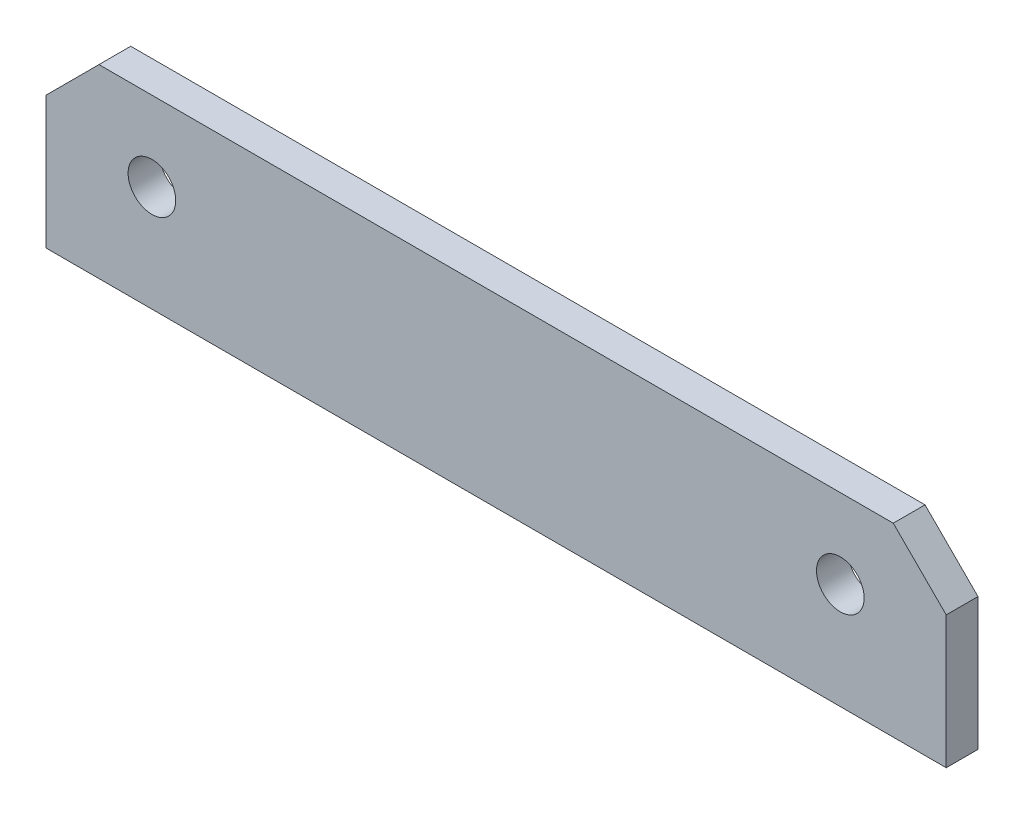
SolidWorks part; units mm, degrees
material "1023 碳钢板 (SS)"
ref_plane "Front Plane" through (0, 0, 0) normal (0, 0, 1) x (1, 0, 0)
ref_plane "Top Plane" through (0, 0, 0) normal (0, 1, 0) x (1, 0, 0)
ref_plane "Right Plane" through (0, 0, 0) normal (1, 0, 0) x (0, 0, -1)
sketch "Sketch1" plane through (0, 0, 0) normal (0, 0, 1) x (1, 0, 0)
  line L0 (-550.1987, 109.2) -> (-651.5, 109.2) construction
  line L1 (-646.5, 109.2) -> (-561.5, 109.2)
  line L2 (-646.5, 109.2) -> (-646.5, 121.7)
  line L3 (-641.5, 126.7) -> (-566.5, 126.7)
  line L4 (-561.5, 109.2) -> (-561.5, 121.7)
  line L5 (-646.5, 121.7) -> (-641.5, 126.7)
  line L6 (-566.5, 126.7) -> (-561.5, 121.7)
  point P1 (-561.5, 126.7)
  point P2 (-646.5, 126.7)
  dimension "D1" = 85
  dimension "D2" = 17.5
  dimension "D3" = 5
extrude "Boss-Extrude1" add sketch "Sketch1" along normal mid plane 3
sketch "Sketch2" plane through (0, 0, 1.5) normal (0, 0, 1) x (1, 0, 0)
  line L0 (-566.5, 126.7) -> (-641.5, 126.7) construction
  circle A0 centre (-636.5, 119.2) radius 2.25
  circle A1 centre (-571.5, 119.2) radius 2.25
  point P4 (-604, 126.7)
  dimension "D1" = 7.5
  dimension "D2" = 32.5
extrude "Cut-Extrude1" cut sketch "Sketch2" against normal blind 3
